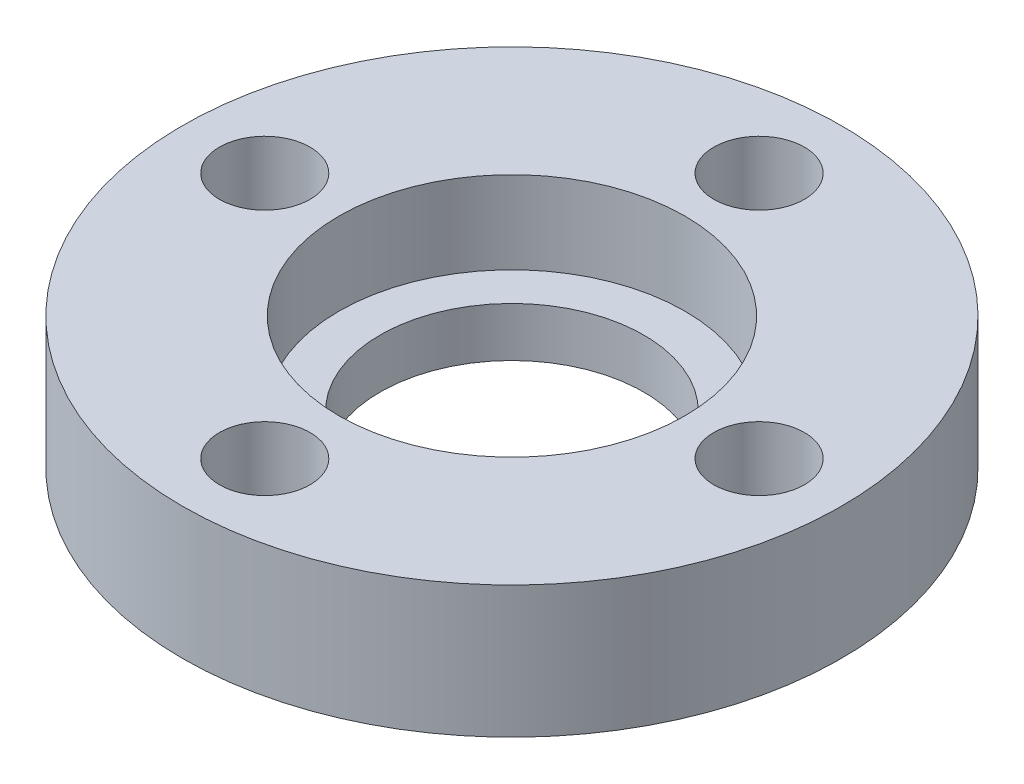
SolidWorks part; units mm, degrees
material "45#"
ref_plane "Front" through (0, 0, 0) normal (0, 0, 1) x (1, 0, 0)
ref_plane "Top" through (0, 0, 0) normal (0, 1, 0) x (1, 0, 0)
ref_plane "Right" through (0, 0, 0) normal (1, 0, 0) x (0, 0, -1)
sketch "Sketch1" plane through (0, 0, 0) normal (0, 1, 0) x (1, 0, 0)
  circle A0 centre (0, 0) radius 40
  circle A1 centre (0, 0) radius 16
  dimension "D1" = 80
  dimension "D2" = 32
extrude "Boss-Extrude1" add sketch "Sketch1" along normal blind 16
sketch "Sketch2" plane through (0, 16, 0) normal (0, 1, 0) x (1, 0, 0)
  circle A0 centre (0, 0) radius 21
  dimension "D1" = 42
extrude "Cut-Extrude1" cut sketch "Sketch2" against normal blind 10
hole_wizard "M10 Clearance Hole1" positions "Sketch5" profile "Sketch6" hole size "M10" standard "GB"
sketch "Sketch5" plane through (0, 16, 0) normal (0, 1, 0) x (1, 0, 0)
  circle A1 centre (0, 0) radius 30
  point P8 (0, 30)
  point P10 (-30, 0)
  point P12 (30, 0)
  point P14 (0, -30)
  dimension "D1" = 60
sketch "Sketch6" plane through (0, 16, 30) normal (1, 0, 0) x (0, 0, 1)
  line L0 (0, 0) -> (0, 32.5547)
  line L1 (0, 32.5547) -> (5.5, 29.25)
  line L2 (5.5, 29.25) -> (5.5, 0)
  line L5 (5.5, 0) -> (0, 0)
  line L10 (0, 32.5547) -> (-5.5, 29.25) construction
  line L11 (0, -6.35) -> (0, 107.95) construction
  dimension "孔直径" = 11
  dimension "孔深度" = 29.25
  dimension "导头角度" = 118
